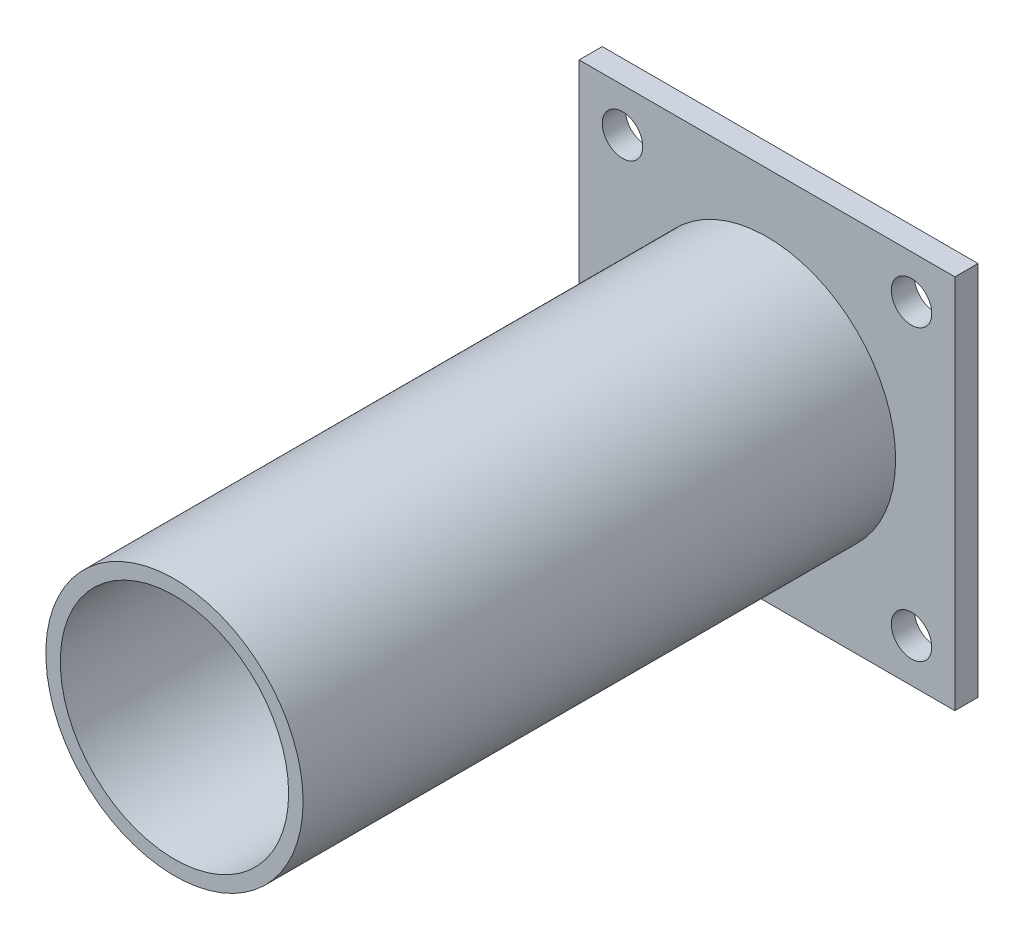
from build123d import *

# Parameters (mm, degrees)
SKETCH_2_W          = 130
SKETCH_2_H          = 130
SKETCH_2_R          = 7
EXTRUDE_1_DEPTH     = 8
SKETCH12_R          = 44.5
SKETCH12_R_2        = 39.5
MEMBER_89X5_1_DEPTH = 205


with BuildPart() as part:
    # 草图2 → 凸台-拉伸1 (new body)
    with BuildSketch(Plane.XY):
        Rectangle(SKETCH_2_W, SKETCH_2_H)
        with Locations((-50, 50)):
            Circle(SKETCH_2_R, mode=Mode.SUBTRACT)
        with Locations(Location((50, 50, 0), (0, 0, 180))):
            Circle(SKETCH_2_R, mode=Mode.SUBTRACT)
        with Locations((50, -50)):
            Circle(SKETCH_2_R, mode=Mode.SUBTRACT)
        with Locations(Location((-50, -50, 0), (0, 0, 180))):
            Circle(SKETCH_2_R, mode=Mode.SUBTRACT)
    extrude(amount=EXTRUDE_1_DEPTH)


with BuildPart() as body_2:
    # Sketch12 → Member 89X5_1 (new body)
    with BuildSketch(Plane.XY.offset(8)):
        Circle(SKETCH12_R)
        Circle(SKETCH12_R_2, mode=Mode.SUBTRACT)
    extrude(amount=MEMBER_89X5_1_DEPTH)


solid = Compound([part.part, body_2.part])
